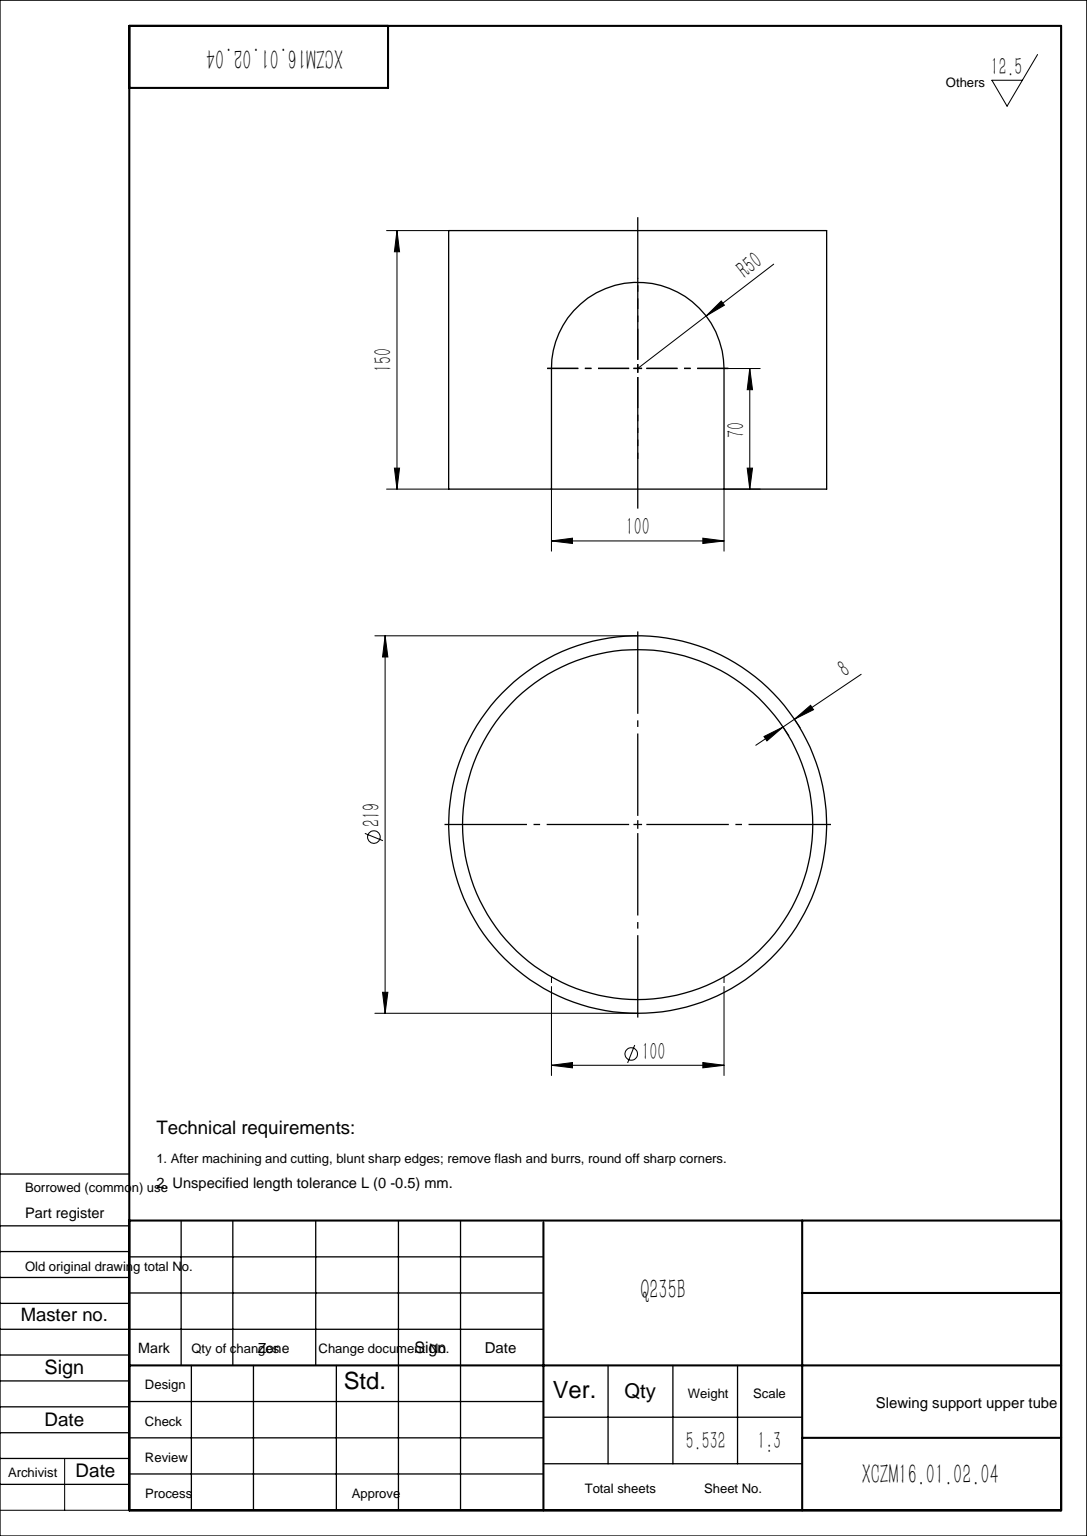
SolidWorks part; units mm, degrees
material "Q235B"
ref_plane "Front Plane" through (0, 0, 0) normal (0, 0, 1) x (1, 0, 0)
ref_plane "Top Plane" through (0, 0, 0) normal (0, 1, 0) x (1, 0, 0)
ref_plane "Right Plane" through (0, 0, 0) normal (1, 0, 0) x (0, 0, -1)
sketch "Sketch1" plane through (0, 0, 0) normal (0, 1, 0) x (1, 0, 0)
  circle A0 centre (0, 0) radius 109.5
  circle A1 centre (0, 0) radius 101.5
  dimension "D1" = 219
  dimension "D2" = 8
extrude "Boss-Extrude1" add sketch "Sketch1" along normal blind 150
sketch "Sketch2" plane through (0, 0, 0) normal (0, 0, 1) x (1, 0, 0)
  line L0 (0, 0) -> (0, 70) construction
  line L1 (-109.5, 0) -> (109.5, 0) construction
  line L2 (-50, 0) -> (-50, 70)
  line L3 (50, 0) -> (50, 70)
  arc A0 (-50, 0) -> (50, 0) centre (0, 0) ccw
  arc A1 (50, 70) -> (-50, 70) centre (0, 70) ccw
  point P4 (0, 35)
  dimension "D2" = 50
  dimension "D1" = 70
extrude "Cut-Extrude1" cut sketch "Sketch2" along normal up to next
